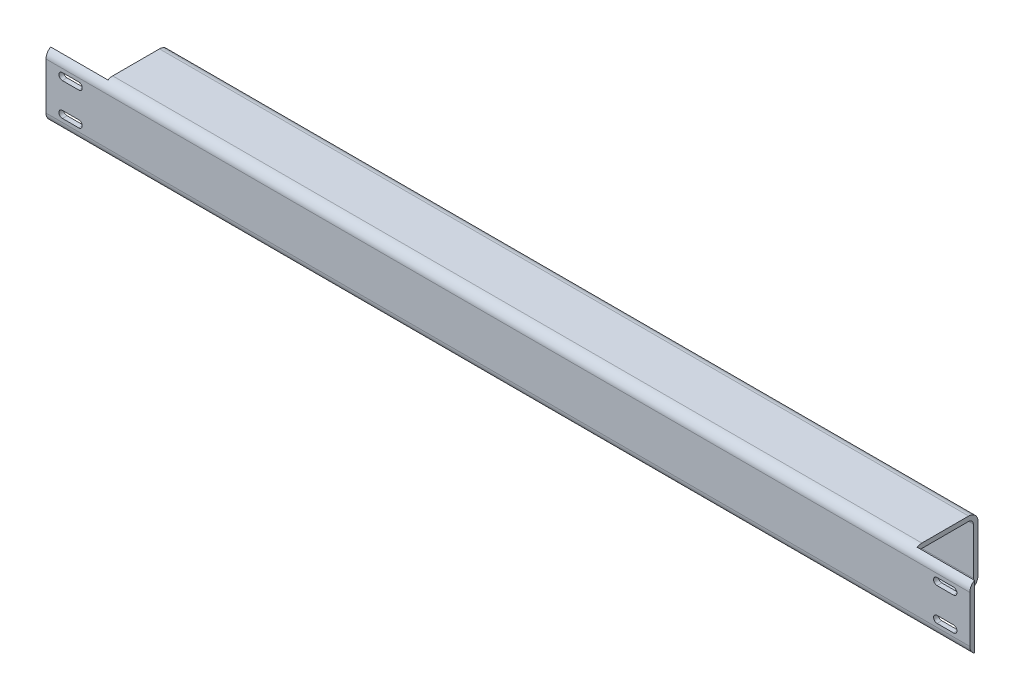
from build123d import *

# Parameters (mm, degrees)
BOSS_EXTRUDE1_DEPTH = 988
BOSS_EXTRUDE2_START = 70
BOSS_EXTRUDE2_DEPTH = 70
BOSS_EXTRUDE3_DEPTH = 70
CUT_EXTRUDE1_DEPTH  = 70


with BuildPart() as part:
    # Sketch1 → Boss-Extrude1 (new body)
    with BuildSketch(Plane(origin=(574, 0, 0), x_dir=(0, 0, -1), z_dir=(1, 0, 0))):
        with BuildLine():
            Line((40, -28.571428571), (40, 28.571428571))
            ThreePointArc((40, 28.571428571), (36.652648928, 36.652648928), (28.571428571, 40))
            Line((28.571428571, 40), (-28.571428571, 40))
            ThreePointArc((-28.571428571, 40), (-36.652648928, 36.652648928), (-40, 28.571428571))
            Line((-40, 28.571428571), (-40, -28.571428571))
            ThreePointArc((-40, -28.571428571), (-36.652648928, -36.652648928), (-28.571428571, -40))
            Line((-28.571428571, -40), (28.571428571, -40))
            ThreePointArc((28.571428571, -40), (36.652648928, -36.652648928), (40, -28.571428571))
        make_face()
        with BuildLine():
            Line((-34.285714286, -28.571428571), (-34.285714286, 28.571428571))
            ThreePointArc((-34.285714286, 28.571428571), (-32.61203875, 32.61203875), (-28.571428571, 34.285714286))
            Line((-28.571428571, 34.285714286), (28.571428571, 34.285714286))
            ThreePointArc((28.571428571, 34.285714286), (32.61203875, 32.61203875), (34.285714286, 28.571428571))
            Line((34.285714286, 28.571428571), (34.285714286, -28.571428571))
            ThreePointArc((34.285714286, -28.571428571), (32.61203875, -32.61203875), (28.571428571, -34.285714286))
            Line((28.571428571, -34.285714286), (-28.571428571, -34.285714286))
            ThreePointArc((-28.571428571, -34.285714286), (-32.61203875, -32.61203875), (-34.285714286, -28.571428571))
        make_face(mode=Mode.SUBTRACT)
    extrude(amount=-BOSS_EXTRUDE1_DEPTH)

    # Sketch2 → Boss-Extrude2 (add)
    with BuildSketch(Plane(origin=(574, 0, 0), x_dir=(0, 0, -1), z_dir=(1, 0, 0)).offset(BOSS_EXTRUDE2_START)):
        with BuildLine():
            Line((-34.285714286, 28.571428571), (-34.285714286, 38.468861758))
            ThreePointArc((-34.285714286, 38.468861758), (-38.468861758, 34.285714286), (-40, 28.571428571))
            Line((-40, 28.571428571), (-40, -28.571428571))
            ThreePointArc((-40, -28.571428571), (-38.468861758, -34.285714286), (-34.285714286, -38.468861758))
            Line((-34.285714286, -38.468861758), (-34.285714286, -28.571428571))
            Line((-34.285714286, -28.571428571), (-34.285714286, 28.571428571))
        make_face()
    extrude(amount=-BOSS_EXTRUDE2_DEPTH)

    # Sketch3 → Boss-Extrude3 (add)
    with BuildSketch(Plane.ZY.offset(414)):
        with BuildLine():
            Line((34.285714286, -28.571428571), (34.285714286, -38.468861758))
            ThreePointArc((34.285714286, -38.468861758), (38.468861758, -34.285714286), (40, -28.571428571))
            Line((40, -28.571428571), (40, 28.571428571))
            ThreePointArc((40, 28.571428571), (38.468861758, 34.285714286), (34.285714286, 38.468861758))
            Line((34.285714286, 38.468861758), (34.285714286, -28.571428571))
        make_face()
    extrude(amount=BOSS_EXTRUDE3_DEPTH)

    # Sketch4 → Cut-Extrude1 (cut)
    with BuildSketch(Plane.XY.offset(40)):
        with BuildLine():
            Line((-464, 24.25), (-444, 24.25))
            ThreePointArc((-444, 24.25), (-439.75, 20), (-444, 15.75))
            Line((-444, 15.75), (-464, 15.75))
            ThreePointArc((-464, 15.75), (-468.25, 20), (-464, 24.25))
        make_face()
        with BuildLine():
            Line((-464, -24.25), (-444, -24.25))
            ThreePointArc((-444, -24.25), (-439.75, -20), (-444, -15.75))
            Line((-444, -15.75), (-464, -15.75))
            ThreePointArc((-464, -15.75), (-468.25, -20), (-464, -24.25))
        make_face()
        with BuildLine():
            Line((604, 24.25), (624, 24.25))
            ThreePointArc((624, 24.25), (628.25, 20), (624, 15.75))
            Line((624, 15.75), (604, 15.75))
            ThreePointArc((604, 15.75), (599.75, 20), (604, 24.25))
        make_face()
        with BuildLine():
            Line((604, -24.25), (624, -24.25))
            ThreePointArc((624, -24.25), (628.25, -20), (624, -15.75))
            Line((624, -15.75), (604, -15.75))
            ThreePointArc((604, -15.75), (599.75, -20), (604, -24.25))
        make_face()
    extrude(amount=-CUT_EXTRUDE1_DEPTH, mode=Mode.SUBTRACT)


solid = part.part
